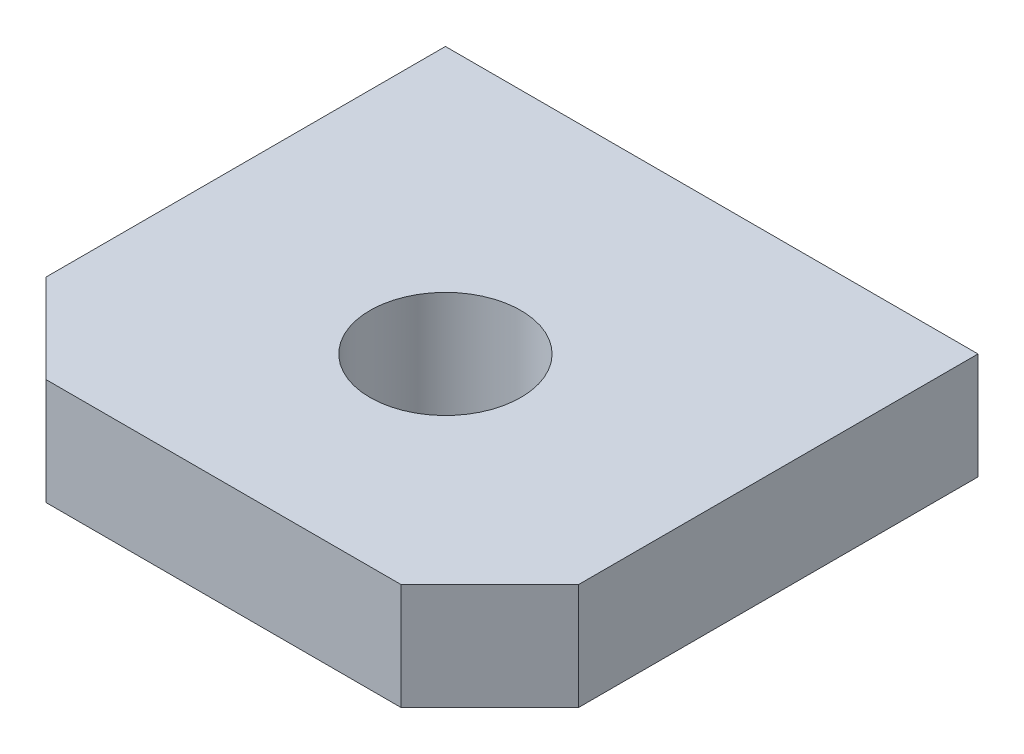
from build123d import *

# Parameters (mm, degrees)
SKETCH1_W           = 60
SKETCH1_H           = 55
SKETCH1_R           = 8.5
BOSS_EXTRUDE1_DEPTH = 12
CHAMFER1_SIZE       = 10


with BuildPart() as part:
    # Sketch1 → Boss-Extrude1 (new body)
    with BuildSketch(Plane(origin=(0, 0, 0), x_dir=(1, 0, 0), z_dir=(0, 1, 0))):
        with Locations((30, -27.5)):
            Rectangle(SKETCH1_W, SKETCH1_H)
        with Locations(Location((30, -30, 0), (0, 0, 270))):
            Circle(SKETCH1_R, mode=Mode.SUBTRACT)
    extrude(amount=BOSS_EXTRUDE1_DEPTH)

    # Chamfer1
    chamfer1_edges = [part.edges().sort_by_distance(p)[0] for p in [
        (60, 6, 55),
        (0, 6, 55),
    ]]
    chamfer(chamfer1_edges, length=CHAMFER1_SIZE)


solid = part.part
